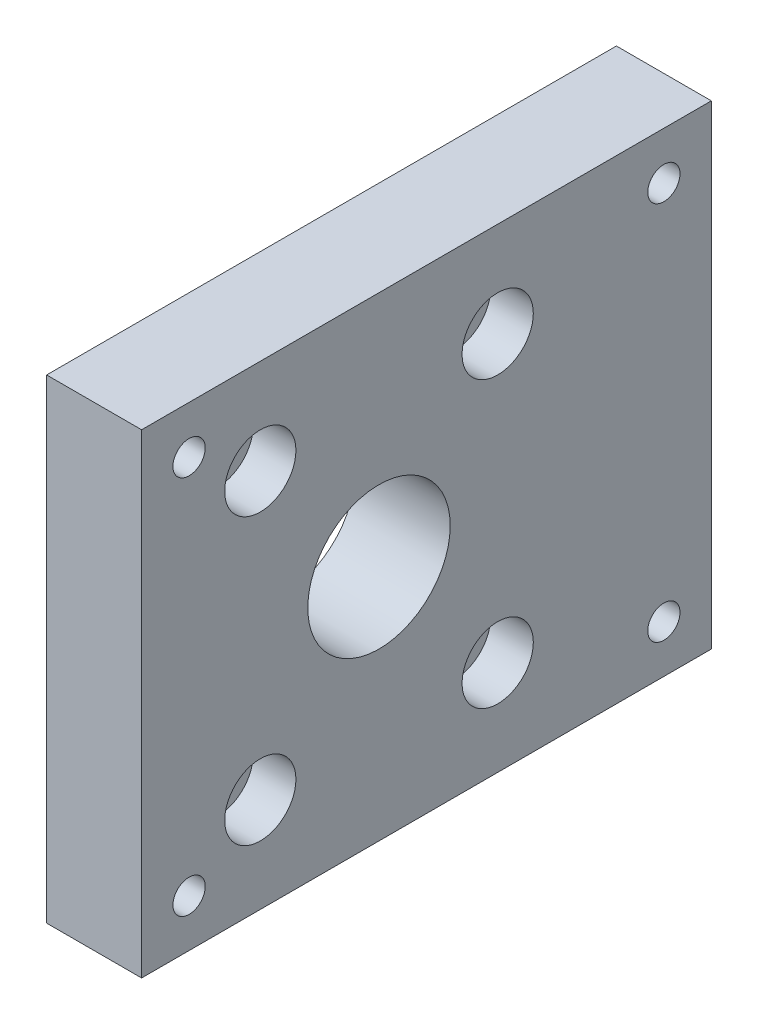
SolidWorks part; units mm, degrees
ref_plane "前视基准面" through (0, 0, 0) normal (0, 0, 1) x (1, 0, 0)
ref_plane "上视基准面" through (0, 0, 0) normal (0, 1, 0) x (1, 0, 0)
ref_plane "右视基准面" through (0, 0, 0) normal (1, 0, 0) x (0, 0, -1)
sketch "草图1" plane through (0, 0, 0) normal (1, 0, 0) x (0, 0, -1)
  line L1 (-60, 50) -> (60, 50)
  line L2 (-60, 50) -> (-60, -50)
  line L3 (-60, -50) -> (60, -50)
  line L4 (60, 50) -> (60, -50)
  line L5 (-60, 50) -> (60, -50) construction
  line L6 (-60, -50) -> (60, 50) construction
  point P0 (0, 0)
  dimension "D1" = 120
  dimension "D2" = 100
extrude "凸台-拉伸1" add sketch "草图1" along normal blind 20
hole_wizard "打孔尺寸(%根据)内六角圆柱头螺钉的类型1" positions "草图2" profile "草图3" counterbore size "M8" standard "GB" end condition through all
sketch "草图2" plane through (20, 0, 0) normal (1, 0, 0) x (0, 0, -1)
  line L0 (-10, 60.9926) -> (-10, 0) construction
  line L1 (-10, 0) -> (49.067, 0) construction
  line L2 (-60, 50) -> (-60, -50) construction
  point P0 (-35, 30)
  point P2 (15, 30)
  point P4 (-35, -30)
  point P6 (15, -30)
  dimension "D1" = 60
  dimension "D2" = 50
  dimension "D3" = 25
sketch "草图3" plane through (20, 30, 35) normal (0, 1, 0) x (0, 0, -1)
  line L0 (0, 0) -> (0, 20)
  line L1 (0, 20) -> (4.5, 20)
  line L3 (4.5, 20) -> (4.5, 9)
  line L4 (4.5, 9) -> (7.5, 9)
  line L5 (7.5, 9) -> (7.5, 0)
  line L7 (7.5, 0) -> (0, 0)
  line L11 (0, -6.35) -> (0, 107.95) construction
  dimension "通孔孔直径" = 9
  dimension "通孔孔深度" = 20
  dimension "柱形沉头孔直径" = 15
  dimension "柱形沉头孔深度" = 9
sketch "草图4" plane through (20, 0, 0) normal (1, 0, 0) x (0, 0, -1)
  line L0 (-35, 30) -> (15, -30) construction
  line L1 (-35, -30) -> (15, 30) construction
  circle A0 centre (-10, 0) radius 15
  dimension "D1" = 30
extrude "切除-拉伸1" cut sketch "草图4" against normal through all
hole_wizard "M8 螺纹孔1" positions "草图5" profile "草图6" tap size "M8" standard "GB" end condition through all
sketch "草图5" plane through (20, 0, 0) normal (1, 0, 0) x (0, 0, -1)
  line L0 (0, 50) -> (0, -50) construction
  line L1 (60, 50) -> (-60, 50) construction
  line L2 (-60, -50) -> (60, -50) construction
  line L4 (60, 0) -> (-70.9342, 0) construction
  line L5 (60, -50) -> (60, 50) construction
  point P0 (-50, 40)
  point P2 (-50, -40)
  point P4 (50, -40)
  point P6 (50, 40)
  dimension "D1" = 100
  dimension "D2" = 80
sketch "草图6" plane through (20, 40, 50) normal (0, 1, 0) x (0, 0, -1)
  line L0 (0, 0) -> (0, 20)
  line L1 (0, 20) -> (3.4, 20)
  line L2 (3.4, 20) -> (3.4, 0)
  line L5 (3.4, 0) -> (0, 0)
  line L11 (0, -6.35) -> (0, 107.95) construction
  dimension "通孔螺纹孔钻头直径" = 6.8
  dimension "通孔螺纹孔钻头深度" = 20
cosmetic thread "孔螺蚊线1" parameters "D2"=8
cosmetic thread "孔螺蚊线2" parameters "D2"=8
cosmetic thread "孔螺蚊线3" parameters "D2"=8
cosmetic thread "孔螺蚊线4" parameters "D2"=8
